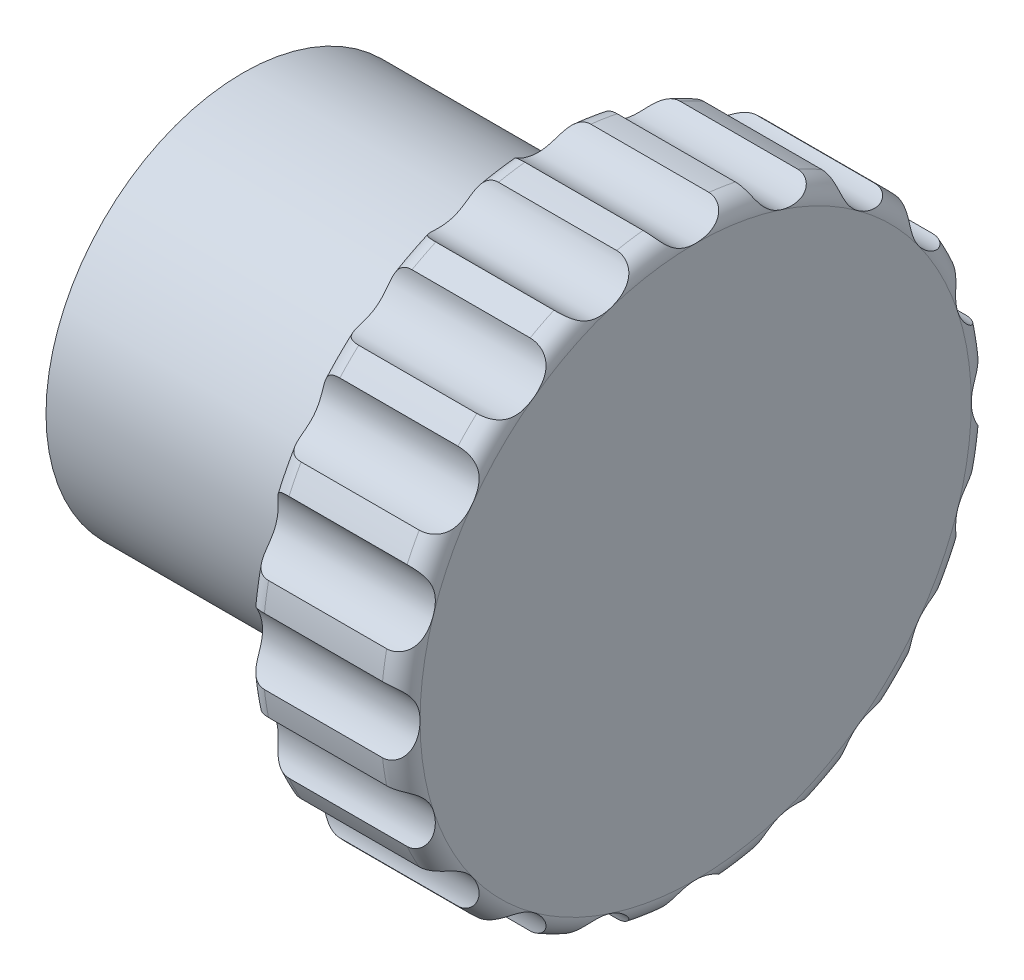
SolidWorks part; units mm, degrees
ref_plane "Front Plane" through (0, 0, 0) normal (0, 0, 1) x (1, 0, 0)
ref_plane "Top Plane" through (0, 0, 0) normal (0, 1, 0) x (1, 0, 0)
ref_plane "Right Plane" through (0, 0, 0) normal (1, 0, 0) x (0, 0, -1)
sketch "Sketch 1" plane through (0, 0, 0) normal (0, 0, 1) x (1, 0, 0)
  line L0 (-9.1026, 0) -> (20.8974, 0) construction
  line L1 (0, 19.8718) -> (0, -20.1282) construction
  line L2 (0, 0) -> (0, 10)
  line L3 (0, 10) -> (15, 10)
  line L4 (15, 10) -> (15, 14)
  line L5 (16, 15) -> (22, 15)
  line L6 (23, 14) -> (23, 0)
  line L7 (23, 0) -> (0, 0)
  arc A0 (22, 15) -> (23, 14) centre (22, 14) cw
  arc A1 (15, 14) -> (16, 15) centre (16, 14) cw
  point P14 (23, 15)
  point P17 (15, 15)
  dimension "D5" = 1
  dimension "D6" = 1
  dimension "D1" = 20
  dimension "D2" = 30
  dimension "D3" = 15
  dimension "D4" = 8
revolve "Revolve 1" add sketch "Sketch 1" angle 360 about L0
sketch "Sketch 2" plane through (23, 0, 0) normal (1, 0, 0) x (0, 0, -1)
  line L0 (0, 18.6081) -> (0, -18.2816) construction
  circle A0 centre (0, 16) radius 2
  circle A1 centre (0, 0) radius 14 construction
  circle A2 centre (4.9443, 15.2169) radius 2
  circle A3 centre (9.4046, 12.9443) radius 2
  circle A4 centre (12.9443, 9.4046) radius 2
  circle A5 centre (15.2169, 4.9443) radius 2
  circle A6 centre (16, 0) radius 2
  circle A7 centre (15.2169, -4.9443) radius 2
  circle A8 centre (12.9443, -9.4046) radius 2
  circle A9 centre (9.4046, -12.9443) radius 2
  circle A10 centre (4.9443, -15.2169) radius 2
  circle A11 centre (0, -16) radius 2
  circle A12 centre (-4.9443, -15.2169) radius 2
  circle A13 centre (-9.4046, -12.9443) radius 2
  circle A14 centre (-12.9443, -9.4046) radius 2
  circle A15 centre (-15.2169, -4.9443) radius 2
  circle A16 centre (-16, 0) radius 2
  circle A17 centre (-15.2169, 4.9443) radius 2
  circle A18 centre (-12.9443, 9.4046) radius 2
  circle A19 centre (-9.4046, 12.9443) radius 2
  circle A20 centre (-4.9443, 15.2169) radius 2
  point P50 (0, 0)
  dimension "D1" = 16
  dimension "D2" = 4
  dimension "D3" = 20
extrude "Cut-Extrude 1" cut sketch "Sketch 2" against normal up to surface (8 mm away) up to face at (15, 0, 10)
